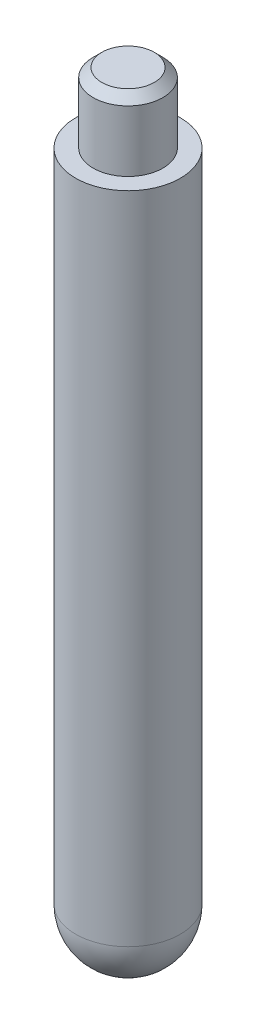
SolidWorks part; units mm, degrees
ref_plane "Front Plane" through (0, 0, 0) normal (0, 0, 1) x (1, 0, 0)
ref_plane "Top Plane" through (0, 0, 0) normal (0, 1, 0) x (1, 0, 0)
ref_plane "Right Plane" through (0, 0, 0) normal (1, 0, 0) x (0, 0, -1)
other "Configuration Table"
sketch "Sketch1" plane through (0, 0, 0) normal (0, 0, 1) x (1, 0, 0)
  line L0 (0, 0) -> (0, 107.9076) construction
  line L1 (0, 90) -> (-4, 90)
  line L2 (-4, 90) -> (-4, 82)
  line L3 (-4, 82) -> (-6, 82)
  line L4 (-6, 82) -> (-6, 7)
  line L5 (0, 90) -> (0, 1)
  arc A0 (-6, 7) -> (0, 1) centre (0, 7) ccw
  dimension "D4" = 6
  dimension "D1" = 4
  dimension "D2" = 6
  dimension "D3" = 75
  dimension "D5" = 8
  dimension "D6" = 90
revolve "Revolve1" add sketch "Sketch1" angle 360 about L0
chamfer "Chamfer1" distance 1 angle 45 1 edges at (0, 90, -4)
